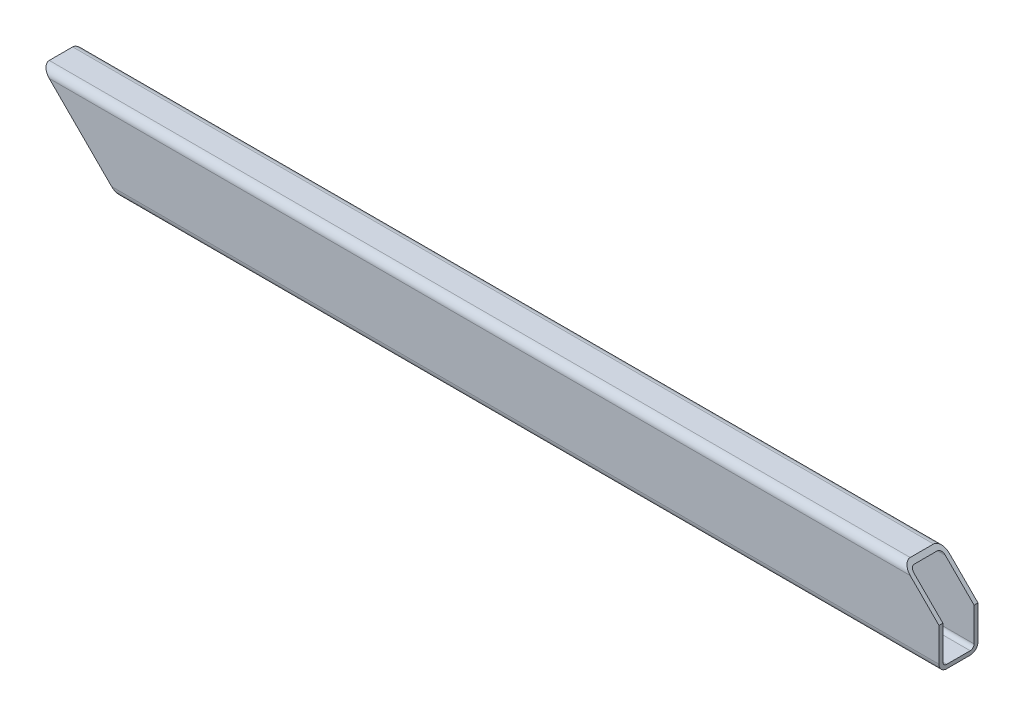
SolidWorks part; units mm, degrees
material "普通碳钢"
ref_plane "前视基准面" through (0, 0, 0) normal (0, 0, 1) x (1, 0, 0)
ref_plane "上视基准面" through (0, 0, 0) normal (0, 1, 0) x (1, 0, 0)
ref_plane "右视基准面" through (0, 0, 0) normal (1, 0, 0) x (0, 0, -1)
sketch3d "3D草图1"
  line L0 (0, 0, 0) -> (1150, 0, 0)
  dimension "D1" = 1150
other "矩形管 100 X 50 X 5(1)"
ref_plane "基准面1" through (0, 0, 0) normal (1, 0, 0) x (0, 0, -1)
sketch "Sketch11" plane through (0, 0, 0) normal (1, 0, 0) x (0, 0, -1)
  line L0 (-15, -45) -> (15, -45)
  line L1 (-20, -40) -> (-20, 40)
  line L2 (15, 45) -> (-15, 45)
  line L3 (20, 40) -> (20, -40)
  line L4 (-15, -50) -> (15, -50)
  line L5 (-25, -40) -> (-25, 40)
  line L6 (15, 50) -> (-15, 50)
  line L7 (25, 40) -> (25, -40)
  arc A0 (25, 40) -> (15, 50) centre (15, 40) ccw
  arc A1 (15, -50) -> (25, -40) centre (15, -40) ccw
  arc A2 (-25, -40) -> (-15, -50) centre (-15, -40) ccw
  arc A3 (-15, 50) -> (-25, 40) centre (-15, 40) ccw
  arc A4 (-15, 45) -> (-20, 40) centre (-15, 40) ccw
  arc A5 (20, 40) -> (15, 45) centre (15, 40) ccw
  arc A6 (15, -45) -> (20, -40) centre (15, -40) ccw
  arc A7 (-20, -40) -> (-15, -45) centre (-15, -40) ccw
  point P0 (0, 50)
  point P1 (25, 0)
  point P2 (0, -50)
  point P3 (-25, 0)
  point P4 (-25, 50)
  point P5 (25, 50)
  point P6 (25, -50)
  point P7 (-25, -50)
  point P8 (0, 0)
  point P33 (0, 0)
  dimension "D1" = 10
  dimension "Thickness" = 5
  dimension "V_leg" = 100
  dimension "H_leg" = 50
sketch "草图2" plane through (0, 75, 25) normal (0, 0, 1) x (1, 0, 0)
  line L0 (0, -25) -> (100, -125)
  line L2 (100, -125) -> (0, -125)
  line L3 (0, -125) -> (0, -25)
  line L4 (1150, -71.9134) -> (1103.0866, -25)
  line L6 (1103.0866, -25) -> (1150, -25)
  line L7 (1150, -25) -> (1150, -71.9134)
  line L9 (1150, -25) -> (0, -25) construction
  line L10 (0, -25) -> (0, -35) construction
  dimension "D1" = 45
  dimension "D2" = 780
extrude "切除-拉伸1" cut sketch "草图2" against normal up to surface (50 mm away) up to face at (575, 0, -25)
